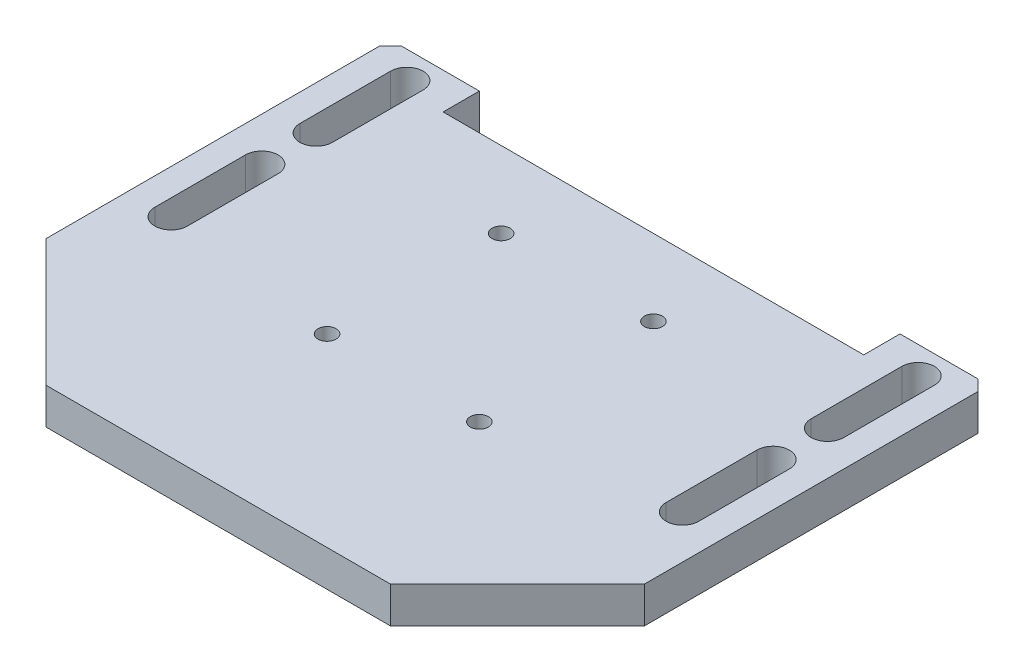
from build123d import *

# Parameters (mm, degrees)
SKETCH_2_W          = 165
SKETCH_2_H          = 130
EXTRUDE_1_DEPTH     = 10
SKETCH_3_W          = 116
SKETCH_3_H          = 10
CUT_EXTRUDE_1_DEPTH = 10
CUT_EXTRUDE_2_DEPTH = 106.50473923
CHAMFER_1_SIZE      = 35
HOLE_WIZARD_M6_1_D  = 5
CHAMFER_3_SIZE      = 3


with BuildPart() as part:
    # 草图2 → 凸台-拉伸1 (new body)
    with BuildSketch(Plane(origin=(0, 0, 0), x_dir=(1, 0, 0), z_dir=(0, 1, 0))):
        Rectangle(SKETCH_2_W, SKETCH_2_H)
    extrude(amount=EXTRUDE_1_DEPTH)

    # 草图3 → 切除-拉伸1 (cut)
    with BuildSketch(Plane(origin=(0, 10, 0), x_dir=(1, 0, 0), z_dir=(0, 1, 0))):
        with Locations((0, 60)):
            Rectangle(SKETCH_3_W, SKETCH_3_H)
    extrude(amount=-CUT_EXTRUDE_1_DEPTH, mode=Mode.SUBTRACT)

    # 草图4 → 切除-拉伸2 (cut, through all)
    with BuildSketch(Plane(origin=(0, 10, 0), x_dir=(1, 0, 0), z_dir=(0, 1, 0))):
        with BuildLine():
            Line((75, 57.5), (75, 32.5))
            ThreePointArc((75, 32.5), (70.5, 28), (66, 32.5))
            Line((66, 32.5), (66, 57.5))
            ThreePointArc((66, 57.5), (70.5, 62), (75, 57.5))
        make_face()
        with BuildLine():
            Line((75, 17.5), (75, -7.5))
            ThreePointArc((75, -7.5), (70.5, -12), (66, -7.5))
            Line((66, -7.5), (66, 17.5))
            ThreePointArc((66, 17.5), (70.5, 22), (75, 17.5))
        make_face()
    cut_extrude_2 = extrude(amount=-CUT_EXTRUDE_2_DEPTH, mode=Mode.SUBTRACT)

    # 倒角1
    chamfer_1_edges = [part.edges().sort_by_distance(p)[0] for p in [
        (82.5, 5, 65),
        (-82.5, 5, 65),
    ]]
    chamfer(chamfer_1_edges, length=CHAMFER_1_SIZE)

    # M6 螺纹孔1 (through all)
    with Locations(Plane(origin=(0, 10, 0), x_dir=(1, 0, 0), z_dir=(0, 1, 0))):
        with Locations((21, -14), (21, 34), (-21, 34), (-21, -14)):
            Hole(HOLE_WIZARD_M6_1_D / 2)

    # 倒角3
    chamfer_3_edges = [part.edges().sort_by_distance(p)[0] for p in [
        (-82.5, 5, -65),
        (82.5, 5, -65),
    ]]
    chamfer(chamfer_3_edges, length=CHAMFER_3_SIZE)

    # 镜向1: 切除-拉伸2 across plane
    add(cut_extrude_2.mirror(Plane(origin=(0, 0, 0), x_dir=(0, 0, 1), z_dir=(1, 0, 0))), mode=Mode.SUBTRACT)


solid = part.part
